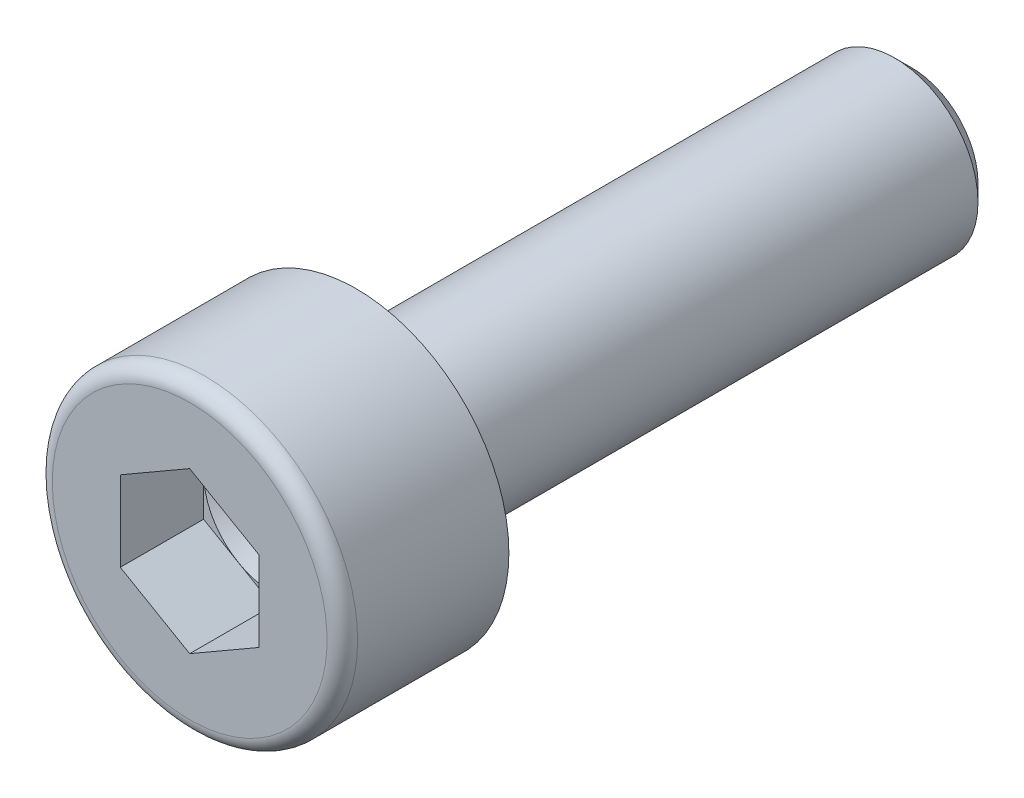
from build123d import *

# Parameters (mm, degrees)
CUT_EXTRUDE1_DEPTH = 1.5
FILLET1_R          = 0.275
CHAMFER1_SIZE      = 0.3
FILLET2_R          = 0.125


with BuildPart() as part:
    # Sketch3 → Revolve1 (revolve)
    with BuildSketch(Plane(origin=(0, 0, 0), x_dir=(0, 0, -1), z_dir=(1, 0, 0)), mode=Mode.PRIVATE) as revolve1_sk:
        Polygon((-3, 0.6), (-3, 2.75), (0, 2.75), (0, 1.5), (10, 1.5), (10, 0.6), align=None)
    revolve(revolve1_sk.sketch.rotate(Axis((0, 0, 3), (0, 0, -1)), 90), axis=Axis((0, 0, 3), (0, 0, -1)))

    # Sketch4 → Cut-Extrude1 (cut)
    with BuildSketch(Plane.XY.offset(3)):
        Polygon((0, 1.443375673), (-1.25, 0.721687836), (-1.25, -0.721687836), (0, -1.443375673), (1.25, -0.721687836), (1.25, 0.721687836), align=None)
    extrude(amount=-CUT_EXTRUDE1_DEPTH, mode=Mode.SUBTRACT)

    # Fillet1
    fillet1_edges = [part.edges().sort_by_distance(p)[0] for p in [
        (-2.75, 0, 3),
    ]]
    fillet(fillet1_edges, radius=FILLET1_R)

    # Chamfer1
    chamfer1_edges = [part.edges().sort_by_distance(p)[0] for p in [
        (-1.5, 0, -10),
    ]]
    chamfer(chamfer1_edges, length=CHAMFER1_SIZE)

    # Cut-Extrude2 cone 1 section (through the dimple's axis) → Cut-Extrude2 (revolve, cut)
    with BuildSketch(Plane(origin=(0, 0, 1.5), x_dir=(0, -1, 0), z_dir=(1, 0, 0))):
        Polygon((0, 0), (1.25, 0), (0, 0.721687836), align=None)
    revolve(axis=Axis((0, 0, 1.5), (0, 0, -1)), mode=Mode.SUBTRACT)

    # Fillet2
    fillet2_edges = [part.edges().sort_by_distance(p)[0] for p in [
        (-1.5, 0, 0),
    ]]
    fillet(fillet2_edges, radius=FILLET2_R)


solid = part.part
